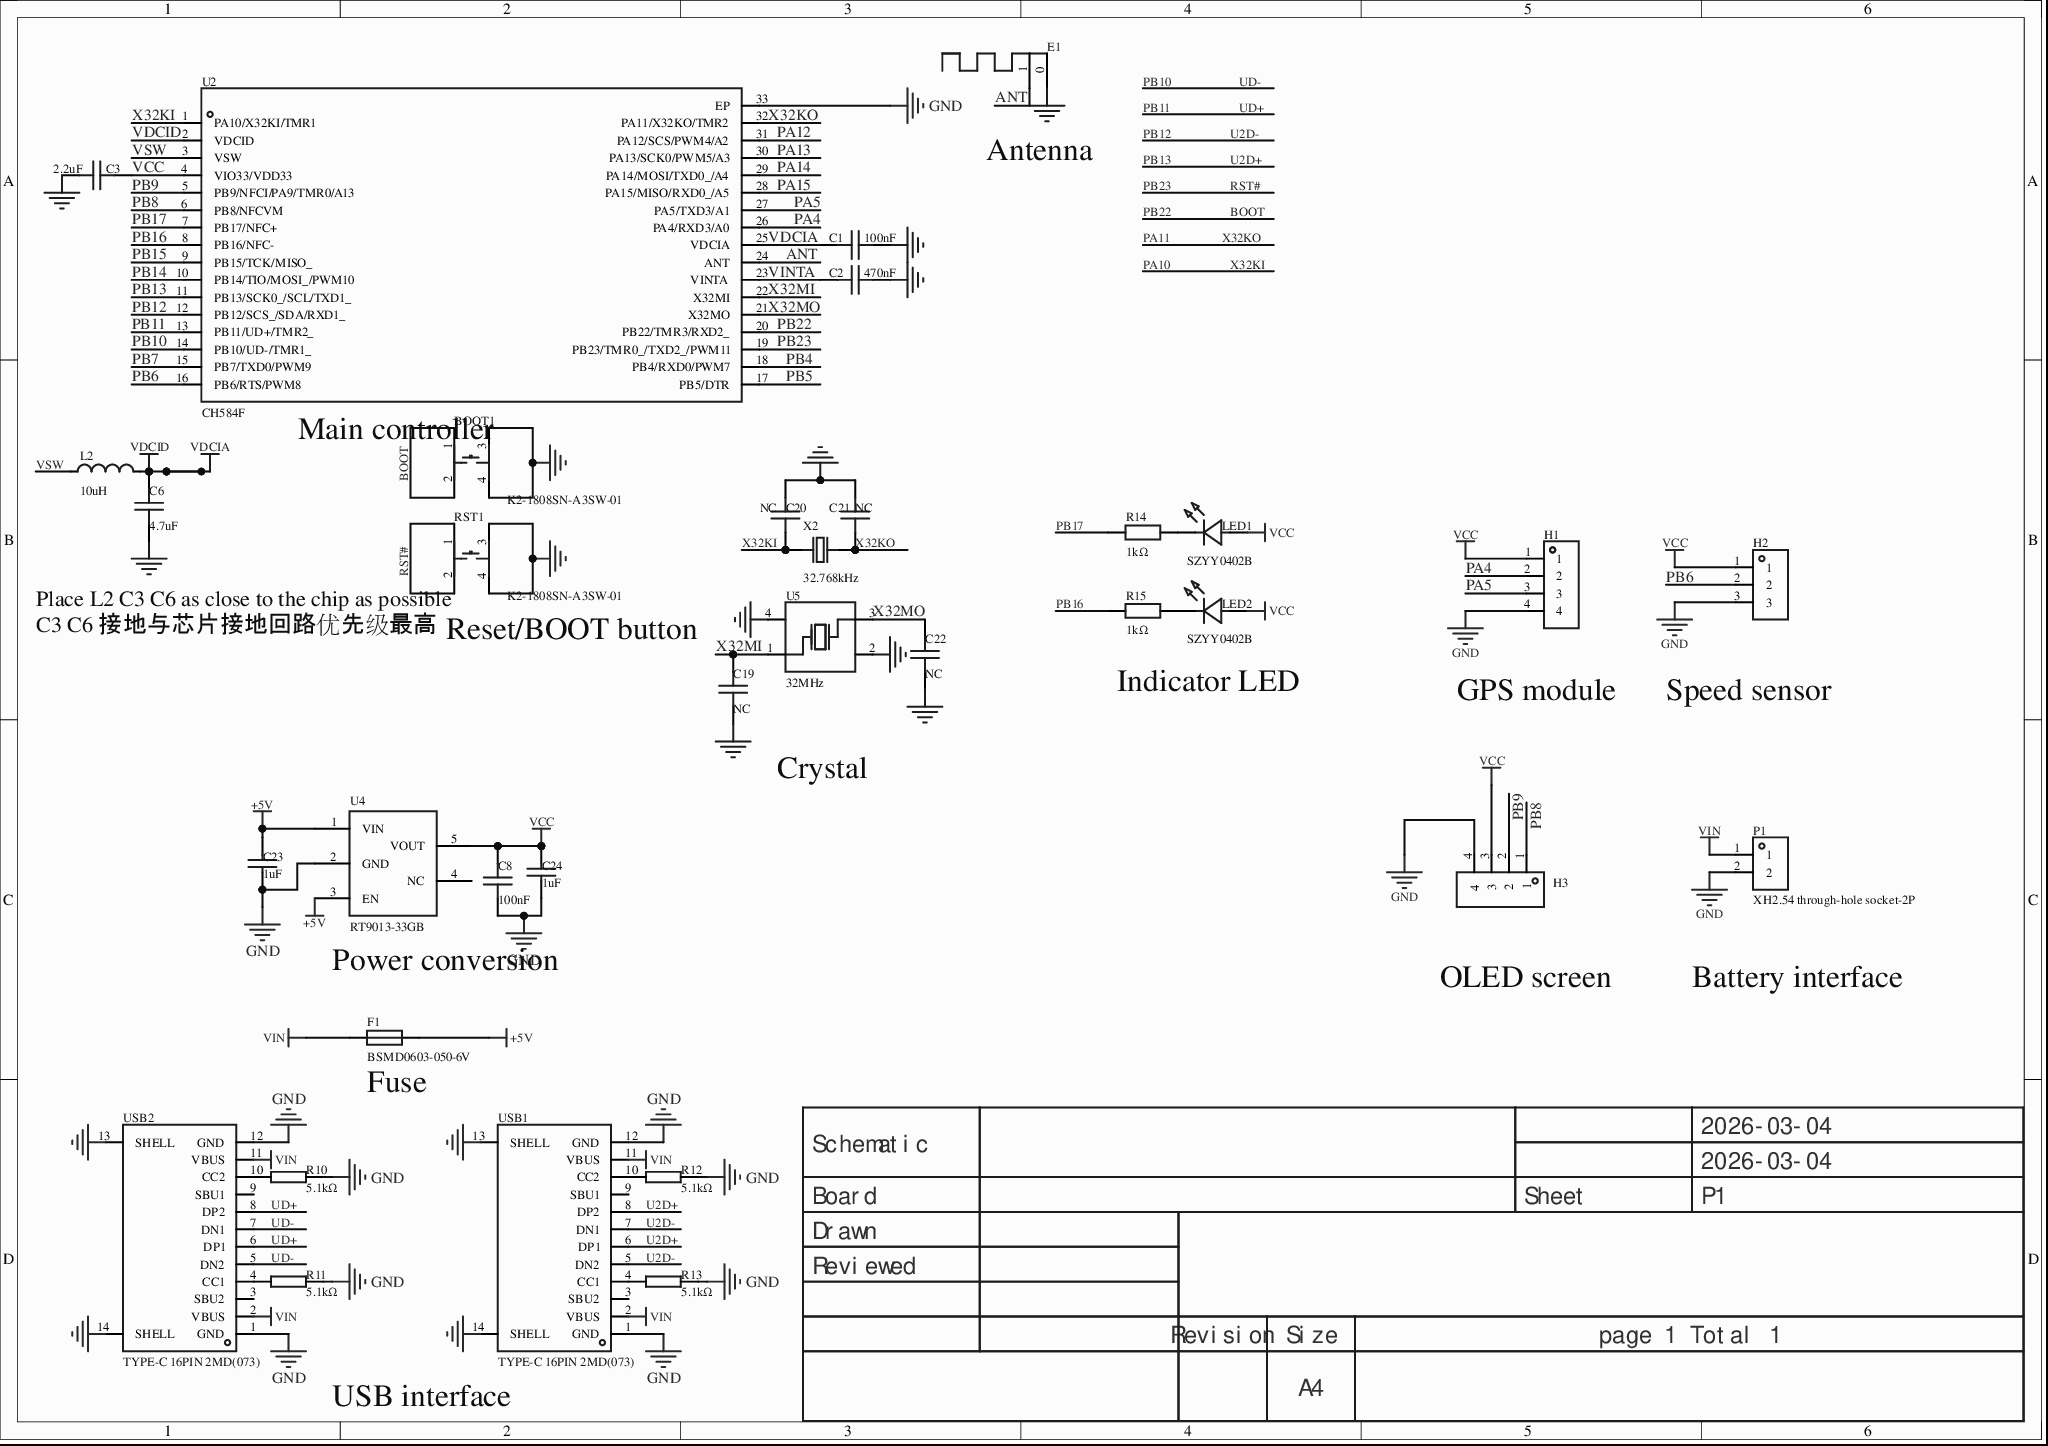
[diagram p0: MISC75430-3.schdoc]
# Altium project MISC75430-2.PrjPcb
1 sheet, 34 parts. Net scope: global (net labels, ports and power ports of the same name join across sheets).
Board file: MISC75430.pcbdoc

## Sheet MISC75430-3.schdoc
size 297 x 209 mm; Version: V1.0; @Project Name: MISC75430; @Page Count: 1; @Update Date: 2026-03-04; @Create Date: 2026-03-04; @Schematic Name: MISC75430; @Page No: 1; @Create Time: 15:42:02; @Update Time: 15:42:02; @Board Name: MISC75430

### Parts
BOOT1  K2-1808SN-A3SW-01  [SW-SMD_4P-L4.2-W3.3-P2.15-LS5.1]
C1  100nF  [0402电容（极简封装）]
C2  470nF  [0402电容（极简封装）]
C3  2.2uF  [0402电容（极简封装）]
C6  4.7uF  [0402电容（极简封装）]
C8  100nF  [0402电容（极简封装）]
C19  NC  [0402电容（极简封装）]
C20  NC  [0402电容（极简封装）]
C21  NC  [0402电容（极简封装）]
C22  NC  [0402电容（极简封装）]
C23  1uF  [0402电容（极简封装）]
C24  1uF  [0402电容（极简封装）]
E1  (no value)  [ANT-F-1-2.4G-1.6mmFR4]
F1  BSMD0603-050-6V  [F0603]
H1  (no value)  [HDR-TH_4P-P2.54-V-F]
H2  (no value)  [HDR-TH_3P-P2.54-V-F]
H3  (no value)  [HDR-TH_4P-P2.54-V-F]
L2  10uH  [IND-SMD_L2.5-W2.0]
LED1  SZYY0402B  [LED0402-RD_BLUE]
LED2  SZYY0402B  [LED0402-RD_BLUE]
P1  XH2.54 through-hole socket-2P  [CONN-TH_XH2.54-2P]
R10  5.1kΩ  [R0402]
R11  5.1kΩ  [R0402]
R12  5.1kΩ  [R0402]
R13  5.1kΩ  [R0402]
R14  1kΩ  [R0603]
R15  1kΩ  [R0603]
RST1  K2-1808SN-A3SW-01  [SW-SMD_4P-L4.2-W3.3-P2.15-LS5.1]
U2  CH584F  [QFN-32_L4.0-W4.0-P0.40-TL-EP2.7]
U4  RT9013-33GB  [SOT-23-5_L3.0-W1.7-P0.95-LS2.8-BR]
U5  32MHz  [CRYSTAL-SMD_4P-L2.0-W1.6-BL-2]
USB1  TYPE-C 16PIN 2MD(073)  [USB-C-SMD_TYPE-C-6PIN-2MD-073]
USB2  TYPE-C 16PIN 2MD(073)  [USB-C-SMD_TYPE-C-6PIN-2MD-073]
X2  32.768kHz  [FC-135R_L3.2-W1.5]

### Nets
+5V: C23.2 F1.2 U4.1(VIN) U4.3(EN)
GND: BOOT1.3 BOOT1.4 C1.2 C2.2 C3.2 C6.1 C8.1 C19.1 C20.2 C21.2 C22.1 C23.1 C24.1 E1.0 H1.4 H2.3 H3.4 P1.2 R10.1 R11.1 R12.1 R13.1 RST1.3 RST1.4 U2.33(EP) U4.2(GND) U5.2(GND) U5.4(GND) USB1.1(GND) USB1.12(GND) USB1.13(SHELL) USB1.14(SHELL) USB2.1(GND) USB2.12(GND) USB2.13(SHELL) USB2.14(SHELL)
VCC: C3.1 C8.2 C24.2 H1.1 H2.1 H3.3 LED1.2(A) LED2.2(A) U2.4(VIO33/VDD33) U4.5(VOUT)
VDCIA: C1.1 C6.2 L2.1 U2.2(VDCID) U2.25(VDCIA)  [also labelled VDCID]
VIN: F1.1 P1.1 USB1.2(VBUS) USB1.11(VBUS) USB2.2(VBUS) USB2.11(VBUS)
ANT: E1.1 U2.24(ANT)
BOOT: BOOT1.1 BOOT1.2 U2.20(PB22/TMR3/RXD2_)  [also labelled PB22]
PA4: H1.2 U2.26(PA4/RXD3/A0)
PA5: H1.3 U2.27(PA5/TXD3/A1)
PA10: C20.1 U2.1(PA10/X32KI/TMR1) X2.1  [also labelled X32KI]
PA11: C21.1 U2.32(PA11/X32KO/TMR2) X2.2  [also labelled X32KO]
PA12: U2.31(PA12/SCS/PWM4/A2)
PA13: U2.30(PA13/SCK0/PWM5/A3)
PA14: U2.29(PA14/MOSI/TXD0_/A4)
PA15: U2.28(PA15/MISO/RXD0_/A5)
PB4: U2.18(PB4/RXD0/PWM7)
PB5: U2.17(PB5/DTR)
PB6: H2.2 U2.16(PB6/RTS/PWM8)
PB7: U2.15(PB7/TXD0/PWM9)
PB8: H3.1 U2.6(PB8/NFCVM)
PB9: H3.2 U2.5(PB9/NFCI/PA9/TMR0/A13)
PB10: U2.14(PB10/UD-/TMR1_) USB2.5(DN2) USB2.7(DN1)  [also labelled UD-]
PB11: U2.13(PB11/UD+/TMR2_) USB2.6(DP1) USB2.8(DP2)  [also labelled UD+]
PB12: U2.12(PB12/SCS_/SDA/RXD1_) USB1.5(DN2) USB1.7(DN1)  [also labelled U2D-]
PB13: U2.11(PB13/SCK0_/SCL/TXD1_) USB1.6(DP1) USB1.8(DP2)  [also labelled U2D+]
PB14: U2.10(PB14/TIO/MOSI_/PWM10)
PB15: U2.9(PB15/TCK/MISO_)
PB16: R15.1 U2.8(PB16/NFC-)
PB17: R14.1 U2.7(PB17/NFC+)
PB23: RST1.1 RST1.2 U2.19(PB23/TMR0_/TXD2_/PWM11)  [also labelled RST#]
VINTA: C2.1 U2.23(VINTA)
VSW: L2.2 U2.3(VSW)
X32MI: C19.2 U2.22(X32MI) U5.1(OSC1)
X32MO: C22.2 U2.21(X32MO) U5.3(OSC2)
NetLED1_1: LED1.1(K) R14.2
NetLED2_1: LED2.1(K) R15.2
NetR10_2: R10.2 USB2.10(CC2)
NetR11_2: R11.2 USB2.4(CC1)
NetR12_2: R12.2 USB1.10(CC2)
NetR13_2: R13.2 USB1.4(CC1)

Not connected (* = marked no-connect by the designer): U4 4(NC)*; USB1 3(SBU2)* 9(SBU1)*; USB2 3(SBU2)* 9(SBU1)*

### Notes on the sheet
- Antenna
- Main controller
- (near RST1) Place L2 C3 C6 as close to the chip as possible
- C3 C6 接地与芯片接地回路优先级最高
- Reset/BOOT button
- Indicator LED
- Crystal
- (near H1) GPS module
- Speed sensor
- Power conversion
- OLED screen
- Battery interface
- (near F1) Fuse
- (near USB1) USB interface
- 2026-03-04
- Schematic
- Board
- Sheet
- P1
- Drawn
- Reviewed
- Revision
- Size
- A4
- page 1 Total 1

### Library data of the parts
BOOT1 RST1 = K2-1808SN-A3SW-01: Contact current: 50mA; rated voltage (DC): 12V; insulation resistance: 100MΩ; mounting: upright SMD; actuation force: 180gf@±30gf; mechanical life: 100000; operating temperature: -25℃~+85℃; switch length: 4.2mm; switch width: 3.25mm; switch height: 2.5mm;; Manufacturer: 韩国韩荣; Circuit: SPST; Actuator Style: Round button; Actuator/Cap Color: Gold; With Lamp: None; Pin Style: SMD tab; Strike Gundam: Without; Symbol: UK-B0267-ZT-SP25Y; AddInBom: yes; ModelId: 101da67941e24d4e9615179a94fc6132; ModelName: SW-SMD_4P-L4.2-W3.3-H2.5-P2.15-LS5.1; ModelTransform: 204.724,127.9525,0,0,0,0,0,0,0; Mechanical Life: 100000; Voltage Rating (AC): -; Power Rating: -; Mounting Style: Upright SMD; IP Rating: -; Diameter: -; Device: K2-1808SN-A3SW-01; LCSC Part Name: 3*4*2.5 贴片开关180G; SupplierPart: C2690012; ManufacturerPart: K2-1808SN-A3SW-01; Supplier Footprint: SMD; JLCPCB Part Class: Extended Part; Datasheet: https://atta.szlcsc.com/upload/public/pdf/source/20180927/C283535_7E7907F3E7B6C1691E1DC87E363D082A.pdf; Supplier: LCSC; ConvertToPcb: yes; FootprintName: SW-SMD_4P-L4.2-W3.3-P2.15-LS5.1; Contact Current: 50mA; Voltage Rating (DC): 12V; Insulation Resistance: 100MΩ; Mounting Sytle: Upright SMD; Operating Force: 180gf@±30gf; Operating Temperature: -25℃~+85℃; Switch Length: 4.2mm; Switch Width: 3.25mm; Switch Height: 2.5mm
C1 C2 = CAP_0402: Symbol: Capacitance; ConvertToPcb: yes; ModelId: 36a51122f27c49738f86b3bfa98863e0; ModelName: C0402_L1.0-W0.5-H0.5; ModelTransform: 39.37,19.685,0,0,0,0,0,0,0; Device: CAP_0402; AddInBom: yes; Supplier Footprint: 0402; FootprintName: 0402 capacitor (simplified package)
  C1: Value: 100nF
  C2: Value: 470nF
C3 C6 C19-C22 = CAP_0402: ConvertToPcb: yes; SymbolName: Capacitance; ModelId: 36a51122f27c49738f86b3bfa98863e0; ModelName: C0402_L1.0-W0.5-H0.5; ModelTransform: 39.37,19.685,0,0,0,0,0,0,0; Device: CAP_0402; AddInBom: yes; Supplier Footprint: 0402; FootprintName: 0402 capacitor (simplified package)
  C3: Value: 2.2uF
  C6: Value: 4.7uF
  C19-C22: Value: NC
C8 = GCM155R71C104KA55J: Capacitance: 100nF; tolerance: ±10%; rated voltage: -; dielectric (temperature coefficient): -;; Manufacturer: muRata(村田); AddInBom: yes; ModelId: 36a51122f27c49738f86b3bfa98863e0; ModelName: C0402_L1.0-W0.5-H0.5; ModelTransform: 39.37,19.685,0,0,0,0,0,0,0; Device: GCM155R71C104KA55J; Symbol: GCM155R71C104KA55J; LCSC Part Name: 100nF ±10%; SupplierPart: C2655418; ManufacturerPart: GCM155R71C104KA55J; Supplier Footprint: 0402; JLCPCB Part Class: Extended Part; Datasheet: https://atta.szlcsc.com/upload/public/pdf/source/20210701/42090801FDE37D0E45AFF657247F4A08.pdf; Supplier: LCSC; ConvertToPcb: yes; FootprintName: 0402 capacitor (simplified package); Value: 100nF; Tolerance: ±10%; Voltage Rated: -; Temperature Coefficient: -
C23 C24 = EMK105BJ105KV-F: Capacitance: 1uF; tolerance: ±10%; rated voltage: 16V; temperature coefficient: X5R;; Manufacturer: TAIYO YUDEN(太诱); AddInBom: yes; ModelId: 36a51122f27c49738f86b3bfa98863e0; ModelName: C0402_L1.0-W0.5-H0.5; ModelTransform: 39.37,19.685,0,0,0,0,0,0,0; Device: EMK105BJ105KV-F; Symbol: EMK105BJ105KV-F; LCSC Part Name: 1uF ±10% 16V; SupplierPart: C92755; ManufacturerPart: EMK105BJ105KV-F; Supplier Footprint: 0402; JLCPCB Part Class: Extended Part; Datasheet: https://atta.szlcsc.com/upload/public/pdf/source/20170103/1483439952086.pdf; Supplier: LCSC; ConvertToPcb: yes; FootprintName: 0402 capacitor (simplified package); Value: 1uF; Tolerance: ±10%; Voltage Rated: 16V; Temperature Coefficient: X5R
E1 = 2.4G天线: Device: 2.4G antenna; AddInBom: yes; ConvertToPcb: yes; SymbolName: 2.4G antenna; FootprintName: ANT-F-1-2.4G-1.6mmFR4
F1 = BSMD0603-050-6V: Withstand voltage (Vmax): 6V; max current (Imax): 40A; hold current (Ihold): 500mA; trip current (Itrip): 1A;; Manufacturer: BHFUSE(佰宏); AddInBom: yes; ModelId: 96143eb6b8924db4a9a1eb67193061e9; ModelName: F0603_L1.7-W0.9-H0.7; ModelTransform: 66.929,35.433,0,0,0,0,0.0005,0.0005,0; Power Dissipation: 500mW; Resistance - Initial (Ri) (Min): 100mΩ; Resistance - Post Trip (R1) (Max): 800mΩ; Symbol: BSMD0603-050-6V; Device: BSMD0603-050-6V; LCSC Part Name: 6V 500mA 0603自恢复; SupplierPart: C883095; ManufacturerPart: BSMD0603-050-6V; Supplier Footprint: 0603; JLCPCB Part Class: Extended library; Datasheet: https://item.szlcsc.com/datasheet/BSMD0603-050-6V/947770.html; Supplier: LCSC; ConvertToPcb: yes; FootprintName: F0603; Voltage - Max: 6V; Current - Max: 40A; Hold Current: 500mA; Trip Current: 1A; Time to Trip(Max): -; Operating Temperature: -40℃~+85℃; Length: 1.85mm; Width: 1.05mm; Height: 1.15mm; Pitch: -
H1 H3 = HDR-F_2.54_1x4P: Symbol: 2.54-1*4P female; ConvertToPcb: yes; ModelId: d187812051054f85879fcaa51a310d8e0819f05c4eef4c71ace90d822a990e87; ModelTransform: 419.6842,98.464,0,0,0,0,0,0,-118.11; Device: HDR-F_2.54_1x4P; AddInBom: yes; SupplierPart: C2718488; Supplier Footprint: 插件; FootprintName: HDR-TH_4P-P2.54-V-F; ModelName: HDR-TH_4P-P2.54-V-F
H2 = HDR-F_2.54_1x3P: Symbol: PM254V-11-03-H85; ConvertToPcb: yes; ModelId: f3b3cc5aae9641bf9e56fc160cef875b0819f05c4eef4c71ace90d822a990e87; ModelName: HDR2.54-F-LI-1X3P; ModelTransform: 299.9994,100,0,0,0,0,0,0,-118.11; Device: HDR-F_2.54_1x3P; AddInBom: yes; SupplierPart: C541850; Supplier Footprint: 插件; FootprintName: HDR-TH_3P-P2.54-V-F
L2 = FTC252012S100MBCA: Inductance: 10uH; tolerance: ±20%; rated current: 1.2A; saturation current (Isat): 1.6A; type: molded inductor;; Manufacturer: cjiang(长江微电); AddInBom: yes; ModelId: 85d117b4abb34d9087271edcd9ba0330; ModelName: IND-SMD_L2.5-W2.0-H1.2; ModelTransform: 99.2124,78.74,0,0,0,0,0,0,0; DC Resistance (DCR): 330mΩ; Symbol: FTC252012S100MBCA; Device: FTC252012S100MBCA; LCSC Part Name: 10uH ±20% 1.6A; SupplierPart: C5832376; ManufacturerPart: FTC252012S100MBCA; Supplier Footprint: SMD,2x2.5mm; JLCPCB Part Class: Extended library; Datasheet: https://atta.szlcsc.com/upload/public/pdf/source/20230602/8FFEDA9C0247A92A0D4B67554BFE4091.pdf; Supplier: LCSC; ConvertToPcb: yes; FootprintName: IND-SMD_L2.5-W2.0; Value: 10uH; Tolerance: ±20%; Rated Current: 1.2A; Saturation Current (Isat): 1.6A; Type: Molded inductor
LED1 LED2 = SZYY0402B: Emitted color: blue; power: -; forward current: 5mA; dominant wavelength: 466nm~469nm; color temperature: -; viewing angle: 120°; packaging: -; operating temperature: -40℃~+85℃;; Manufacturer: yongyu(永裕光电); AddInBom: yes; ModelId: 080bb9bd520f4b34ac21e218e7b036d6; ModelName: LED0402_L1.0-W0.5-H0.2; ModelTransform: 40.1574,19.685,0,0,0,0,0,-0.0005,0; Symbol: SZYY0402B; Device: SZYY0402B; LCSC Part Name: 蓝灯; SupplierPart: C434447; ManufacturerPart: SZYY0402B; Supplier Footprint: 0402; JLCPCB Part Class: Extended library; Datasheet: https://atta.szlcsc.com/upload/public/pdf/source/20210222/C434447_30232BB6183B52026028ECA50B9DAB35.pdf; Supplier: LCSC; ConvertToPcb: yes; FootprintName: LED0402-RD_BLUE; Emitted Color: Blue; Power Dissipation: -; Forward Current: 5mA; Dominant Wavelength: 466nm~469nm; Peak Wavelength: -; Color Temperature: -; Viewing Angle: 120°; Mounting Sytle: -; Operating Temperature: -40℃~+85℃
P1 = XH2.54直插座-2P: AddInBom: yes; ModelId: c3cc11bd8b8748c1ae6bc231aac3a1ff0819f05c4eef4c71ace90d822a990e87; ModelTransform: 296.889,230.315,0,0,0,0,0,26.653,-137.795; Symbol: XH2.54 through-hole socket-2P; Device: XH2.54 through-hole socket-2P; LCSC Part Name: XH2.54直插座-2P; SupplierPart: C9900016957; ManufacturerPart: XH2.54直插座-2P; Supplier Footprint: XH2.54-2; JLCPCB Part Class: Extended Part; Supplier: LCSC; ConvertToPcb: yes; FootprintName: CONN-TH_XH2.54-2P; ModelName: CONN-TH_XH2.54-2P
R10-R13 = 0402WGF1001TCE: Resistor type: thick-film resistor; resistance: 1kΩ; tolerance: ±1%; power: 62.5mW; max working voltage: 50V; temperature coefficient: ±100ppm/℃;; Manufacturer: UNI-ROYAL(厚声); Symbol: RES; AddInBom: yes; ModelId: 98c88bc2b9094f218f3a3e30a7012738; ModelName: R0402_L1.0-W0.5-H0.4; ModelTransform: 39.37,19.685,0,0,0,0,0,0,0; Value: 5.1kΩ; Device: 0402WGF1001TCE; LCSC Part Name: 1kΩ ±1% 62.5mW 厚膜电阻; ManufacturerPart: 0402WGF1001TCE; Supplier Footprint: 0402; JLCPCB Part Class: Basic Part; Datasheet: https://atta.szlcsc.com/upload/public/pdf/source/20200306/C422600_1E6D84923E4A46A82E41ADD87F860B5C.pdf; Supplier: LCSC; ConvertToPcb: yes; FootprintName: R0402; Type: Thick-film resistor; Tolerance: ±1%; Power(Watts): 62.5mW; Overload Voltage (Max): 50V; Temperature Coefficient: ±100ppm/℃; Operating Temperature Range: -55℃~+155℃
R14 R15 = 0603WAF1001T5E: Resistor type: thick-film resistor; resistance: 1kΩ; tolerance: ±1%; power: 100mW; max working voltage: 75V; temperature coefficient: ±100ppm/℃;; Manufacturer: UNI-ROYAL(厚声); AddInBom: yes; ModelId: fc143cca1e79419f9cd78b61e9279f08; ModelTransform: 31.8897,63.7794,0,90,0,0,0,0,0; Symbol: 0603WAF1001T5E; Device: 0603WAF1001T5E; LCSC Part Name: 1kΩ ±1% 100mW 厚膜电阻; SupplierPart: C21190; ManufacturerPart: 0603WAF1001T5E; Supplier Footprint: 0603; JLCPCB Part Class: Basic library; Datasheet: https://atta.szlcsc.com/upload/public/pdf/source/20200306/C422600_1E6D84923E4A46A82E41ADD87F860B5C.pdf; Supplier: LCSC; ConvertToPcb: yes; FootprintName: R0603; ModelName: R0603; Type: Thick-film resistor; Value: 1kΩ; Tolerance: ±1%; Power(Watts): 100mW; Overload Voltage (Max): 75V; Temperature Coefficient: ±100ppm/℃; Operating Temperature Range: -55℃~+155℃
U2 = CH584F: CH585 is a RISC-V MCU/SoC with integrated BLE wireless communication and high-speed USB and NFC. It integrates a 2Mbps low-power Bluetooth BLE communication module, a USB full-speed controller and transceiver, a USB high-speed controller and transceiver (480Mbps), an NFC near-field communication wireless interface, a segment LCD driver module, an LED matrix interface, 2 SPI, 4 UART, 14-channel ADC, touch-key detection module and other rich peripheral resources.; Manufacturer: WCH(南京沁恒); AddInBom: yes; ModelId: 1e9eca8b25044b9fa4f766d7d1391f8f0819f05c4eef4c71ace90d822a990e87; ModelTransform: 158.267,158.267,0,0,0,0,0,0,0; Symbol: CH584F; Device: CH584F; LCSC Part Name: 集成BLE无线通讯和高速USB及NFC的RISC-V MCU/SoC; SupplierPart: C42381468; ManufacturerPart: CH584F; Supplier Footprint: QFN-32(4x4); JLCPCB Part Class: Extended Part; Datasheet: https://item.szlcsc.com/datasheet/CH584F/44296585.html; Supplier: LCSC; ConvertToPcb: yes; FootprintName: QFN-32_L4.0-W4.0-P0.40-TL-EP2.7; ModelName: QFN-32_L4.0-W4.0-P0.40-TL-EP2.7
U4 = RT9013-33GB: Output type: fixed; output polarity: positive; output channels: 1; max input voltage: 5.5V; output voltage: 3.3V; dropout: 400mV@(500mA); quiescent (ground) current: -; output current: 500mA; PSRR: 50dB@(10kHz); noise: -; features: -;; Manufacturer: RICHTEK(台湾立锜); AddInBom: yes; ModelId: 0a2a1b8f50944f73965918ad6e5fe167; ModelName: SOT-23-5_L2.9-W1.6-H1.1-LS2.8-P0.95; ModelTransform: 114.173,109.636,0,180,0,0,-0.863,0.863,0; Number of Outputs: 1; Device: RT9013-33GB; Symbol: RT9013-33GB; LCSC Part Name: Vin=5.5V Vout=3.3V 500mA 50dB@(10kHz); SupplierPart: C47773; ManufacturerPart: RT9013-33GB; Supplier Footprint: SOT-23-5; JLCPCB Part Class: Extended Part; Datasheet: https://atta.szlcsc.com/upload/public/pdf/source/20150504/1457707282459.pdf; Supplier: LCSC; ConvertToPcb: yes; FootprintName: SOT-23-5_L3.0-W1.7-P0.95-LS2.8-BR; Output Type: Fixed; Output Polarity: Positive; Maximum Input Voltage: 5.5V; Output Voltage: 3.3V; Dropout Voltage: 400mV@(500mA); Quiescent Current (Ground Current): -; Output Current: 500mA; Power Supply Rejection Ratio (PRSS): 50dB@(10kHz); Noise: -; Feature: -
U5 = XL7EL89COI-111YLC-32M: Crystal type: SMD crystal; frequency: 32MHz; frequency deviation at room temperature: ±10ppm; load capacitance: 12pF; frequency stability: ±20ppm;; Manufacturer: YXC(扬兴晶振); AddInBom: yes; ModelId: 3c7217722bdc4daeae1fd6f7f164cfcf; ModelTransform: 78.74,62.992,0,0,0,0,0,0,0; Symbol: XL7EL89COI-111YLC-32M; Device: XL7EL89COI-111YLC-32M; LCSC Part Name: YSX211SL 32MHZ 4P 2016 12PF ±10PPM -40~85℃ (±20PPM); SupplierPart: C2965584; ManufacturerPart: XL7EL89COI-111YLC-32M; Supplier Footprint: SMD2016-4P; JLCPCB Part Class: Extended library; Datasheet: https://item.szlcsc.com/datasheet/XL7EL89COI-111YLC-32M/3357720.html; Supplier: LCSC; ConvertToPcb: yes; FootprintName: CRYSTAL-SMD_4P-L2.0-W1.6-BL-2; ModelName: CRYSTAL-SMD_4P-L2.0-W1.6-BL-2; Type: SMD crystal; Value: 32MHz; Normal temperature Frequency Tolerance: ±10ppm; Load Capacitance: 12pF; Frequency Stability: ±20ppm; Equivalent Series Resistance(ESR): -; Operating Temperature: -40℃~+85℃
USB1 USB2 = TYPE-C 16PIN 2MD(073): Connector type: Type-C; protocol standard: USB 3.1; gender: female; mounting: horizontal SMD; contacts: 16P; ports: 1; rated current - power: 3A; operating temperature: -25℃~+85℃;; Manufacturer: SHOU HAN(首韩); Current Rating - Power (Max): 5A; AddInBom: yes; ModelId: 3a41b9ec9b654a0fad4d118405ec6290; ModelTransform: 351.9678,298.4246,0,0,0,0,0,-47.244,-35.433; Protocol Standard: USB 3.1; Number of Ports: 1; Voltage Rating: 5V; Connect-Disconnect Life: 5 thousand cycles; Detection color: Black; Standard: -; Mounting Style: Horizontal SMD; Operating Temperature Range: -25℃~+85℃; Symbol: TYPE-C 16PIN 2MD(073); Device: TYPE-C 16PIN 2MD(073); Supplier: LCSC; Supplier Part: C2765186; Manufacturer Part: TYPE-C 16PIN 2MD(073); JLCPCB Part Class: Extended library; LCSC Part Name: Type-C 母 卧贴; Supplier Footprint: SMD; Datasheet: https://atta.szlcsc.com/upload/public/pdf/source/20250506/FFB74EDFDFA0AC372CE4A8E4F739CCEF.pdf; ConvertToPcb: yes; FootprintName: USB-C-SMD_TYPE-C-6PIN-2MD-073; ModelName: USB-C-SMD_TYPE-C-6PIN-2MD-073; Connector Type: Type-C; Gender: Female; Mounting Type: Horizontal SMD; Number of Contacts: 16P; Current Rating-Power: 3A; Supplementary Features: -; Center Height: -; Length: -; Operating Temperature: -25℃~+85℃
X2 = Q13FC13500004_C32346: Crystal type: SMD crystal; frequency: 32.768kHz; frequency deviation at room temperature: ±20ppm; load capacitance: 12.5pF;; Manufacturer: EPSON(爱普生); Symbol: Q13FC1350000400; AddInBom: yes; ModelId: 751105e878f044059ef0ee72de95f96e; ModelTransform: 125.984,59.055,0,0,0,0,0,0,0; Equivalent Series Resistance (ESR): 70kΩ; Device: Q13FC13500004_C32346; LCSC Part Name: 32.768kHz ±20ppm 12.5pF; SupplierPart: C32346; ManufacturerPart: Q13FC13500004; Supplier Footprint: SMD3215-2P; JLCPCB Part Class: Basic library; Datasheet: https://atta.szlcsc.com/upload/public/pdf/source/20240418/0E0FF5F0356BA3753F616001439D1416.pdf; Supplier: LCSC; ConvertToPcb: yes; FootprintName: FC-135R_L3.2-W1.5; ModelName: FC-135R_L3.2-W1.5; Crystal Type: SMD crystal; Value: 32.768kHz; Normal temperature Frequency Tolerance: ±20ppm; Load Capacitor: 12.5pF; Operating Temperature: -40℃~+85℃